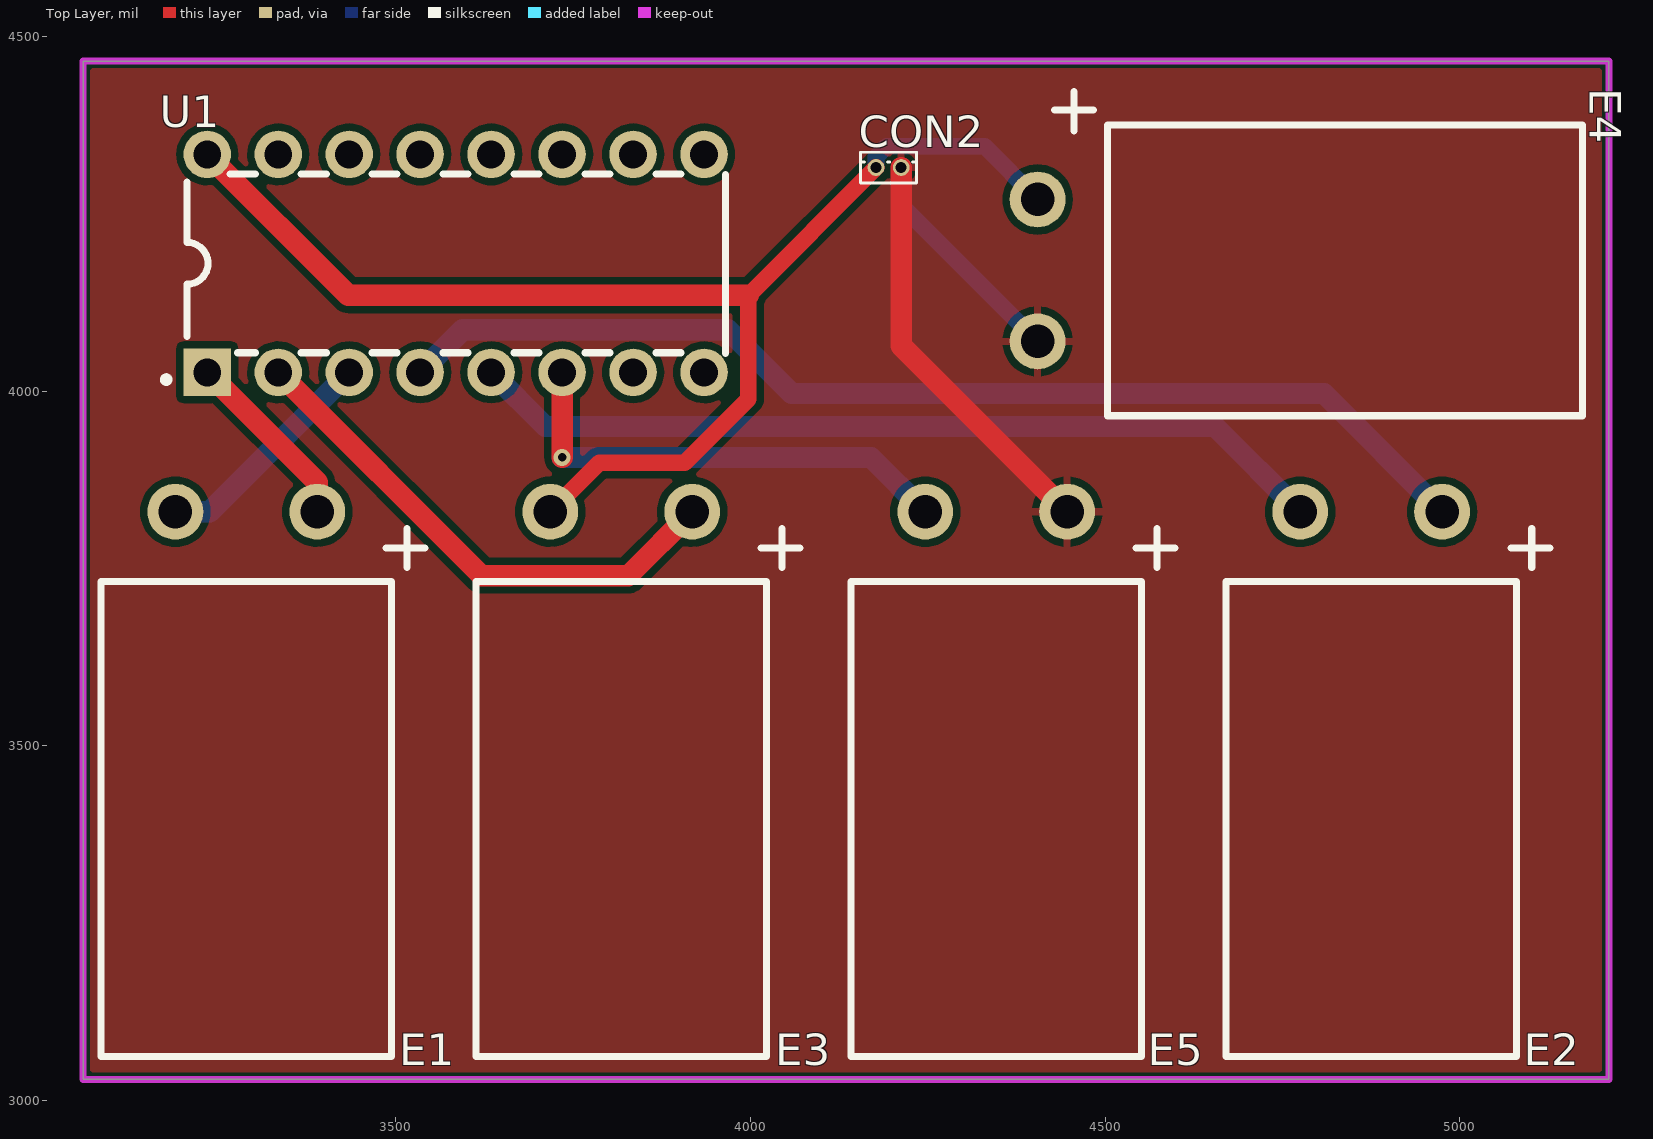
[diagram p0: Top Layer view]
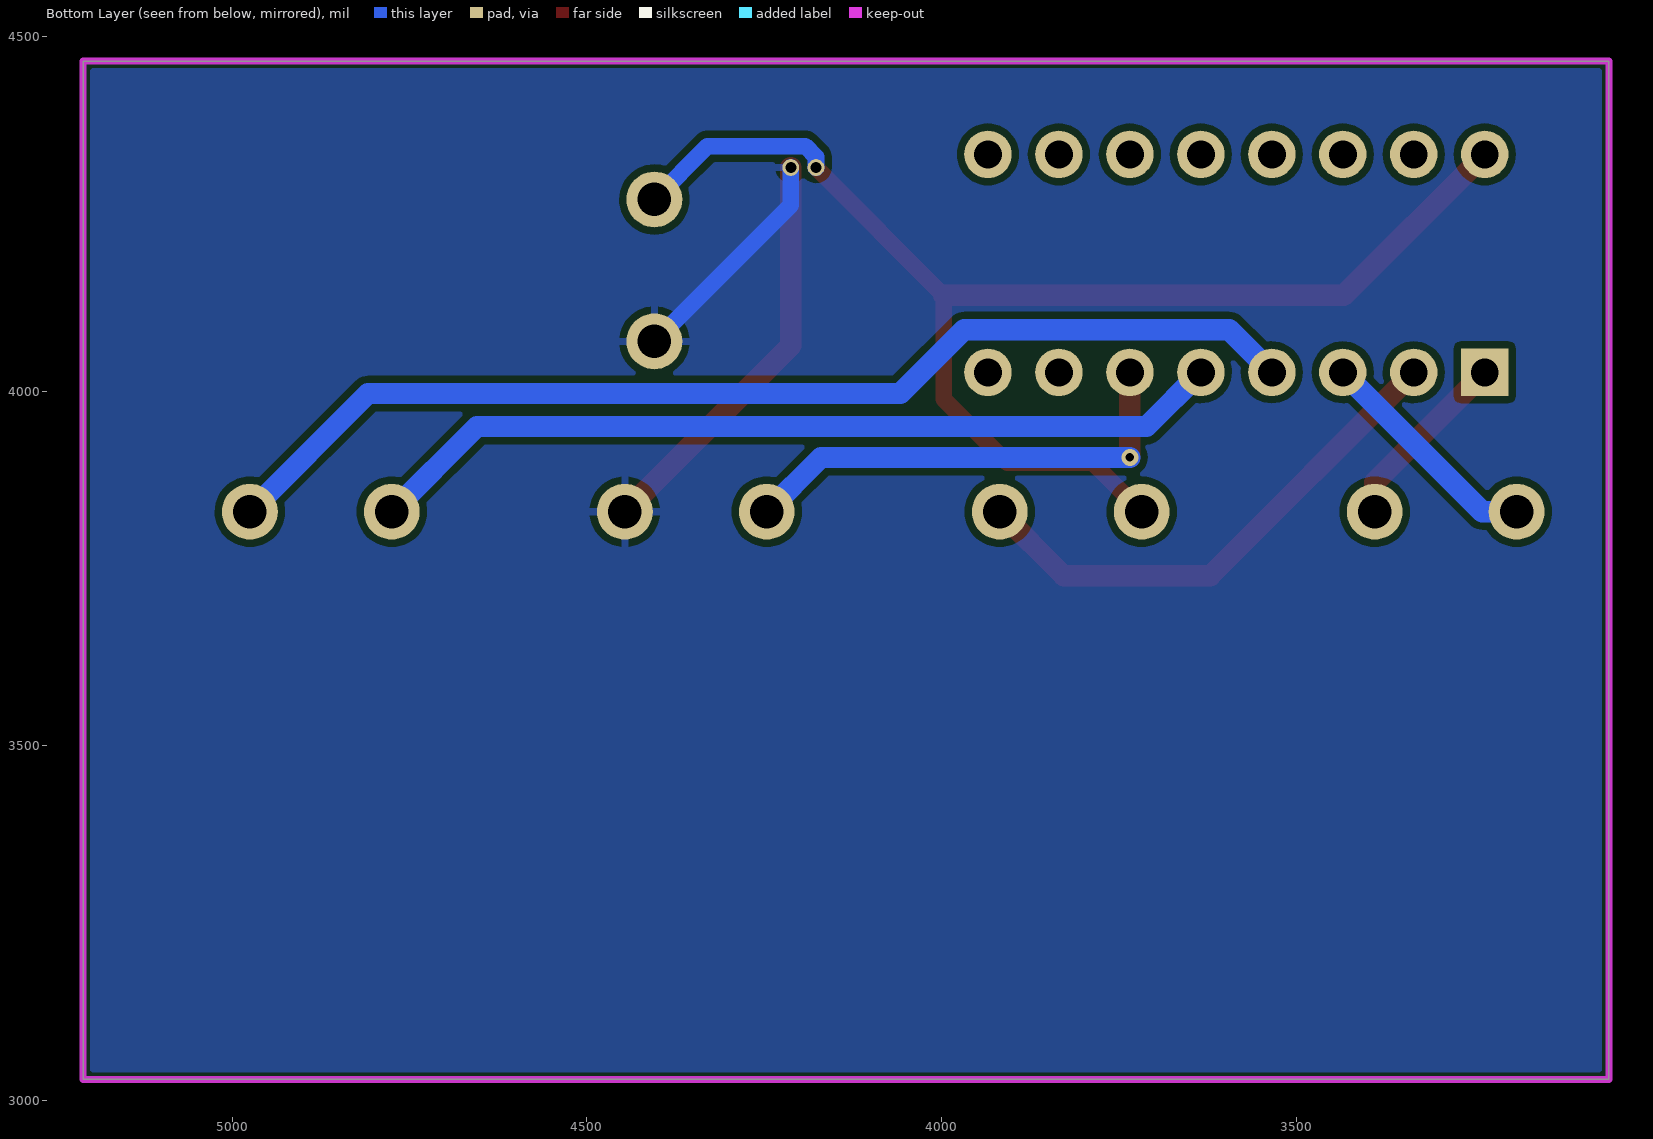
[diagram p1: Bottom Layer view, seen from below]
# Altium PCB MISC51987.pcbdoc
Units mil, origin at the board's own origin, x right, y up, seen from the top; angles counter-clockwise.
Board outline 2150 x 1435 mil, 2 copper layers (Top Layer, Bottom Layer), stack 62.206 mil thick; 7 components, 10 nets, 28 pads, 1 vias.

## Layer stack, top to bottom
Top Solder Mask Layer: solder mask 0.394, Dk 3.3
Top Layer: signal copper 1.379
Dielectric1: surface 59.449, FR4, Dk 4.5
Bottom Layer: signal copper 1.378
Bottom Solder Mask Layer: solder mask 0.394, Dk 3.3

## Board outline
3060,4465 3060,3030 5210,3030 5210,4465

## Design rules (kind name [scope] priority, off if disabled: settings)
BoardOutlineClearance copperThickness2oz_1 [All] p2 off: genericclearance=7.99 ignorepadtopadclearanceinfootprint=FALSE except(0: Arc-SplitContinuation Track-SplitContinuation SMDPad-SplitContinuation THPad-SplitContinuation Via-SplitContinuation Fill-SplitContinuation Region-SplitContinuation Poly-SplitContinuation Text-SplitContinuation Hole-SplitContinuation; 5.98: Arc-CutoutEdge Track-CutoutEdge SMDPad-CutoutEdge THPad-CutoutEdge Via-CutoutEdge Text-CutoutEdge; 6.89: Hole-OutlineEdge Hole-CutoutEdge; 10: Poly-OutlineEdge Poly-CutoutEdge; 11.81: Arc-OutlineEdge Track-OutlineEdge SMDPad-OutlineEdge THPad-OutlineEdge Via-OutlineEdge Fill-OutlineEdge Region-OutlineEdge Text-OutlineEdge Fill-CutoutEdge Region-CutoutEdge)
BoardOutlineClearance Plane_innerPlane_1 [All] p4 off: genericclearance=4.02 ignorepadtopadclearanceinfootprint=FALSE except(0: Arc-SplitContinuation Track-SplitContinuation SMDPad-SplitContinuation THPad-SplitContinuation Via-SplitContinuation Fill-SplitContinuation Region-SplitContinuation Poly-SplitContinuation Text-SplitContinuation Hole-SplitContinuation; 5.98: Arc-CutoutEdge Track-CutoutEdge SMDPad-CutoutEdge THPad-CutoutEdge Via-CutoutEdge Text-CutoutEdge; 6.89: Hole-OutlineEdge Hole-CutoutEdge; 10: Poly-OutlineEdge Poly-CutoutEdge; 11.81: Arc-OutlineEdge Track-OutlineEdge SMDPad-OutlineEdge THPad-OutlineEdge Via-OutlineEdge Fill-OutlineEdge Region-OutlineEdge Text-OutlineEdge Fill-CutoutEdge Region-CutoutEdge)
BoardOutlineClearance Copper_copperRegion_1 [All] p6 off: genericclearance=4.02 ignorepadtopadclearanceinfootprint=FALSE except(0: Arc-SplitContinuation Track-SplitContinuation SMDPad-SplitContinuation THPad-SplitContinuation Via-SplitContinuation Fill-SplitContinuation Region-SplitContinuation Poly-SplitContinuation Text-SplitContinuation Hole-SplitContinuation; 5.98: Arc-CutoutEdge Track-CutoutEdge SMDPad-CutoutEdge THPad-CutoutEdge Via-CutoutEdge Text-CutoutEdge; 6.89: Hole-OutlineEdge Hole-CutoutEdge; 10: Poly-OutlineEdge Poly-CutoutEdge; 11.81: Arc-OutlineEdge Track-OutlineEdge SMDPad-OutlineEdge THPad-OutlineEdge Via-OutlineEdge Fill-OutlineEdge Region-OutlineEdge Text-OutlineEdge Fill-CutoutEdge Region-CutoutEdge)
BoardOutlineClearance copperThickness1oz_1 [All] p8: genericclearance=4.02 ignorepadtopadclearanceinfootprint=FALSE except(0: Arc-SplitContinuation Track-SplitContinuation SMDPad-SplitContinuation THPad-SplitContinuation Via-SplitContinuation Fill-SplitContinuation Region-SplitContinuation Poly-SplitContinuation Text-SplitContinuation Hole-SplitContinuation; 5.98: Arc-CutoutEdge Track-CutoutEdge SMDPad-CutoutEdge THPad-CutoutEdge Via-CutoutEdge Text-CutoutEdge; 6.89: Hole-OutlineEdge Hole-CutoutEdge; 10: Poly-OutlineEdge Poly-CutoutEdge; 11.81: Arc-OutlineEdge Track-OutlineEdge SMDPad-OutlineEdge THPad-OutlineEdge Via-OutlineEdge Fill-OutlineEdge Region-OutlineEdge Text-OutlineEdge Fill-CutoutEdge Region-CutoutEdge)
Clearance copperThickness2oz [All] p1 off: gap=7.99 ignorepadtopadclearanceinfootprint=FALSE except(5.98: SMDPad-Track SMDPad-SMDPad THPad-Track SMDPad-THPad THPad-THPad Track-Via SMDPad-Via THPad-Via Via-Via Fill-SMDPad Region-SMDPad Fill-THPad Region-THPad Fill-Via Region-Via Fill-Fill Fill-Region Region-Region Arc-Track Arc-SMDPad Arc-THPad Arc-Via Fill-Arc Region-Arc Arc-Arc Text-Track SMDPad-Text Text-THPad Text-Via Fill-Text Region-Text Arc-Text Text-Text; 6.89: Hole-Track Hole-SMDPad Hole-THPad Hole-Via Fill-Hole Region-Hole Hole-Arc Hole-Text; 10: Poly-Track Poly-SMDPad Poly-THPad Poly-Via Poly-Fill Poly-Region Poly-Poly Poly-Arc Poly-Text Poly-Hole; 11.81: Fill-Track Region-Track)
Clearance Plane_innerPlane [All] p3 off: gap=4.02 ignorepadtopadclearanceinfootprint=FALSE except(5.98: SMDPad-Track SMDPad-SMDPad THPad-Track SMDPad-THPad THPad-THPad Track-Via SMDPad-Via THPad-Via Via-Via Fill-SMDPad Region-SMDPad Fill-THPad Region-THPad Fill-Via Region-Via Fill-Fill Fill-Region Region-Region Arc-Track Arc-SMDPad Arc-THPad Arc-Via Fill-Arc Region-Arc Arc-Arc Text-Track SMDPad-Text Text-THPad Text-Via Fill-Text Region-Text Arc-Text Text-Text; 6.89: Hole-Track Hole-SMDPad Hole-THPad Hole-Via Fill-Hole Region-Hole Hole-Arc Hole-Text; 10: Poly-Track Poly-SMDPad Poly-THPad Poly-Via Poly-Fill Poly-Region Poly-Poly Poly-Arc Poly-Text Poly-Hole; 11.81: Fill-Track Region-Track)
Clearance Copper_copperRegion [All] p5 off: gap=4.02 ignorepadtopadclearanceinfootprint=FALSE except(5.98: SMDPad-Track SMDPad-SMDPad THPad-Track SMDPad-THPad THPad-THPad Track-Via SMDPad-Via THPad-Via Via-Via Fill-SMDPad Region-SMDPad Fill-THPad Region-THPad Fill-Via Region-Via Fill-Fill Fill-Region Region-Region Arc-Track Arc-SMDPad Arc-THPad Arc-Via Fill-Arc Region-Arc Arc-Arc Text-Track SMDPad-Text Text-THPad Text-Via Fill-Text Region-Text Arc-Text Text-Text; 6.89: Hole-Track Hole-SMDPad Hole-THPad Hole-Via Fill-Hole Region-Hole Hole-Arc Hole-Text; 10: Poly-Track Poly-SMDPad Poly-THPad Poly-Via Poly-Fill Poly-Region Poly-Poly Poly-Arc Poly-Text Poly-Hole; 11.81: Fill-Track Region-Track)
Clearance copperThickness1oz [All] p7: gap=4.02 ignorepadtopadclearanceinfootprint=FALSE except(5.98: SMDPad-Track SMDPad-SMDPad THPad-Track SMDPad-THPad THPad-THPad Track-Via SMDPad-Via THPad-Via Via-Via Fill-SMDPad Region-SMDPad Fill-THPad Region-THPad Fill-Via Region-Via Fill-Fill Fill-Region Region-Region Arc-Track Arc-SMDPad Arc-THPad Arc-Via Fill-Arc Region-Arc Arc-Arc Text-Track SMDPad-Text Text-THPad Text-Via Fill-Text Region-Text Arc-Text Text-Text; 6.89: Hole-Track Hole-SMDPad Hole-THPad Hole-Via Fill-Hole Region-Hole Hole-Arc Hole-Text; 10: Poly-Track Poly-SMDPad Poly-THPad Poly-Via Poly-Fill Poly-Region Poly-Poly Poly-Arc Poly-Text Poly-Hole; 11.81: Fill-Track Region-Track)
DiffPairsRouting differentialPair [All] p1: maxlimit=6 minlimit=6 mostfreqgap=6 toplayer_minwidth=5 toplayer_prefwidth=10 toplayer_maxwidth=100 toplayer_mingap=6 toplayer_prefgap=6 toplayer_maxgap=6 bottomlayer_minwidth=5 bottomlayer_prefwidth=10 bottomlayer_maxwidth=100 bottomlayer_mingap=6 bottomlayer_prefgap=6 bottomlayer_maxgap=6 maxuncoupledlength=10
HoleToHoleClearance otherClearance [All] p1: gap=11.81 allowstackedmicrovias=TRUE
Length netLength [All] p1: minlimit=0 maxlimit=0
PasteMaskExpansion pasteMaskExpansion [All] p1: expansion=0
PlaneConnect innerPlane [All] p1: planeconnectstyle=Relief reliefexpansion=20 reliefentries=4 reliefconductorwidth=10 reliefairgap=10
PolygonConnect copperRegion [All] p1: connectstyle=Relief reliefconductorwidth=10 reliefentries=4 polygonreliefangle="90 Angle" airgapwidth=10 via.connectstyle=Relief via.reliefconductorwidth=10 via.reliefentries=4 via.polygonreliefangle="90 Angle" via.airgapwidth=10
RoutingVias viaSize [All] p1: holewidth=12.01 width=24.02 viastyle="Through Hole" minholewidth=11.81 minwidth=19.68 maxholewidth=248.03 maxwidth=393.7
SolderMaskExpansion solderMaskExpansion [IsVia] p1: expansion=-1000 istentingtop=TRUE
SolderMaskExpansion solderMaskExpansion [All] p2: expansion=2.01 istentingtop=FALSE
Width copperThickness2oz_2 [All] p1 off: maxlimit=100 minlimit=8 preferedwidth=10
Width copperThickness1oz_2 [All] p2: maxlimit=100 minlimit=5 preferedwidth=30

## Components (designator, comment, footprint, x,y, rotation, side; value= is the part's Value field where it differs from the comment)
CON2 "" SIP-2_L2.0-W1.1-P0.90-D0.3 4195,4315 r0 top
E1 "1uf" CAP-TH_L17.0-W10.4-P5.08_CDK11A_470UF 3290,3830 r180 top
E2 "1uf" CAP-TH_L17.0-W10.4-P5.08_CDK11A_470UF 4875,3830 r180 top
E3 "1uf" CAP-TH_L17.0-W10.4-P5.08_CDK11A_470UF 3818.33,3830 r180 top
E4 "1uf" CAP-TH_L17.0-W10.4-P5.08_CDK11A_470UF 4405,4170 r270 top
E5 "1uf" CAP-TH_L17.0-W10.4-P5.08_CDK11A_470UF 4346.67,3830 r180 top
U1 "MAX232IDR-TD" DIP-16_L19.7-W6.6-P2.54-LS10.9-BL 3585,4180 r0 top

## Footprints (in the part's own frame and the unit in brackets; to place one, negate y for a bottom-side part, rotate by r counter-clockwise, add the part's x,y. Pads: shape width x height; smd on the part's side, far side on the other; paste and mask are expansions set on the pad)
CAP-TH_L17.0-W10.4-P5.08_CDK11A_470UF [mm]
  round 2 hole 1.2: 1(-2.54,0) 2(2.54,0)
  silkscreen extent -6.4,0.6 5.2,19.5
DIP-16_L19.7-W6.6-P2.54-LS10.9-BL [mm]
  rect 1.7x1.7 hole 1: 1(-8.89,-3.9)
  round 1.7 hole 1: 2(-6.35,-3.9) 3(-3.81,-3.9) 4(-1.27,-3.9) 5(1.27,-3.9) 6(3.81,-3.9) 7(6.35,-3.9) 8(8.89,-3.9) 9(8.89,3.9) 10(6.35,3.9) 11(3.81,3.9) 12(1.27,3.9) 13(-1.27,3.9) 14(-3.81,3.9) 15(-6.35,3.9) 16(-8.89,3.9)
  silkscreen extent -10.46,-4.26 9.66,3.2
SIP-2_L2.0-W1.1-P0.90-D0.3 [mm]
  round 0.6 hole 0.4 paste+0 mask+0.05: 1(-0.45,0) 2(0.45,0)
  silkscreen extent -1,-0.55 1,0.55

## Via types
v1: diameter 24.02, hole 12, Top Layer to Bottom Layer, 1 vias

## Nets (pads, with @x,y where several pads share a name; then routed paths per layer and width w, separated by ;. In a path a pad name is that pad's centre, name@x,y a point inside that pad or via, vN(x,y) a via of type N, cw(c..) or ccw(c..) an arc to the next point about the centre after c; other vN are vias at no path point)
$1N412: E2.2 U1.5 | length 1221.4
  Bottom Layer w30: U1.5 3711.46,3950 4655,3950 E2.2
$1N421: E2.1 U1.4 | length 1571.1
  Bottom Layer w30: U1.4 3595,4086.46 3968.54,4086.46 4058.54,3996.46 4808.54,3996.46 E2.1
$1N455: E1.2 U1.3 | length 326.4
  Bottom Layer w30: E1.2 3238.54,3830 U1.3
$1N459: E1.1 U1.1 | length 260.7
  Top Layer w30: U1.1 3390,3871.46 E1.1
$1N615: E3.1 U1.2 | length 739.3
  Top Layer w30: U1.2 3621.46,3740 3828.33,3740 E3.1
$1N627: E5.2 U1.6 | length 663.3
  Top Layer w30: v1(3735,3906.46) U1.6
  Bottom Layer w30: v1(3735,3906.46) 4170.21,3906.46 E5.2
GND: CON2.2 E4.2 E5.1 | length 906.6
  Top Layer w30: CON2.2 4212.72,4063.95 E5.1
  Bottom Layer w23.62: CON2.2 4212.72,4262.28 E4.2
RS232IN: U1.13
TTLOUT: U1.12
VCC: CON2.1 E3.2 E4.1 U1.16 | length 1869.9
  Top Layer w23.62: E3.2 3787.28,3898.95 3907.28,3898.95 3997.28,3988.95 3997.28,4135 CON2.1
  Top Layer w30: U1.16 3433.54,4135 3997.28,4135
  Bottom Layer w23.62: CON2.1 4177.28,4330 4192.28,4345 4330,4345 E4.1
pads on no net: U1.7 U1.8 U1.9 U1.10 U1.11 U1.14 U1.15

## Polygon pours and split planes (outlines as drawn)
GND on Top Layer (solid, remove dead copper, pour order 0): 3000,4525 3000,3000 5260,3000 5260,4525
GND on Bottom Layer (solid, remove dead copper, pour order 2): 3010,4505 3010,3000 5260,3000 5260,4505

## Keep-outs
Board Outline Layer:
  the board outline again, w10